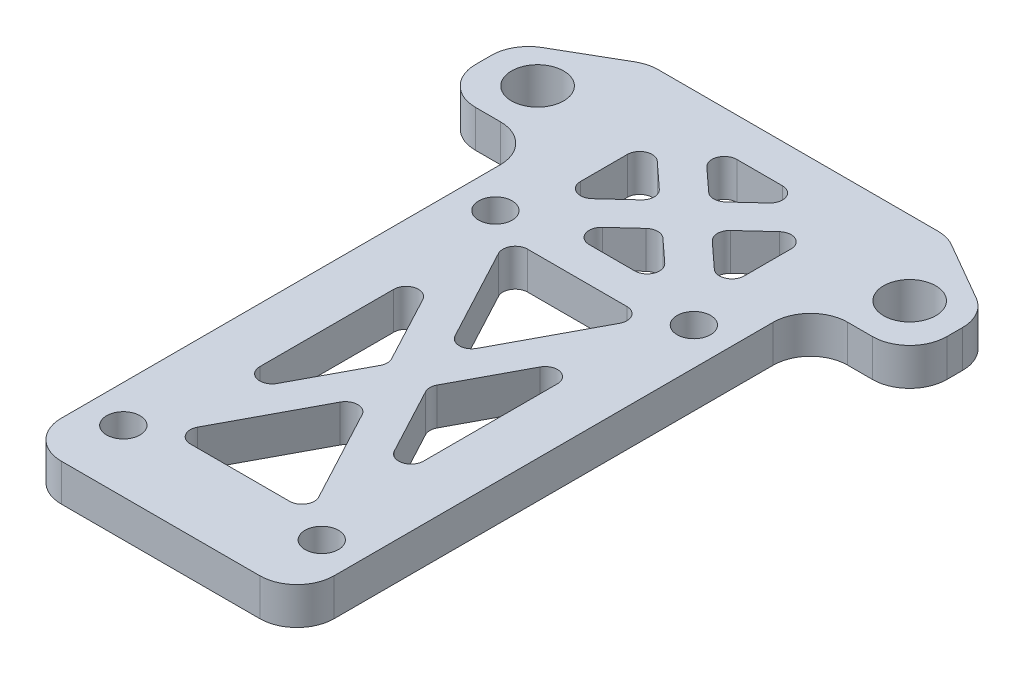
from build123d import *

# Parameters (mm, degrees)
SKETCH_1_R          = 2.1
SKETCH_1_R_2        = 1.35
EXTRUDE_1_DEPTH     = 3
CUT_EXTRUDE_1_DEPTH = 50.306794664
FILLET_R3_R         = 3
FILLET_R1_R         = 1


with BuildPart() as part:
    # 草图1 → 凸台-拉伸1 (new body)
    with BuildSketch(Plane(origin=(0, 0, 0), x_dir=(1, 0, 0), z_dir=(0, 1, 0))):
        Polygon((-12.07179677, 6), (-19, 2), (-19, -4), (-11, -4), (-11, -45.4), (11, -45.4), (11, -4), (19, -4), (19, 2), (12.07179677, 6), align=None)
        with Locations(Location((-15, 0, 0), (0, 0, 270))):
            Circle(SKETCH_1_R, mode=Mode.SUBTRACT)
        with Locations(Location((15, 0, 0), (0, 0, 270))):
            Circle(SKETCH_1_R, mode=Mode.SUBTRACT)
        with Locations(Location((-8, -10.4, 0), (0, 0, 270))):
            Circle(SKETCH_1_R_2, mode=Mode.SUBTRACT)
        with Locations(Location((-8, -40.4, 0), (0, 0, 270))):
            Circle(SKETCH_1_R_2, mode=Mode.SUBTRACT)
        with Locations(Location((8, -10.4, 0), (0, 0, 90))):
            Circle(SKETCH_1_R_2, mode=Mode.SUBTRACT)
        with Locations(Location((8, -40.4, 0), (0, 0, 90))):
            Circle(SKETCH_1_R_2, mode=Mode.SUBTRACT)
    extrude(amount=EXTRUDE_1_DEPTH)

    # 草图2 → 切除-拉伸1 (cut, through all)
    with BuildSketch(Plane(origin=(0, 3, 0), x_dir=(1, 0, 0), z_dir=(0, 1, 0))):
        Polygon((-6.6, 1.112582185), (-6.6, -7.212582185), (-2.069298303, -3.05), align=None)
        Polygon((-4.406892174, 2.9), (0, -1.148832185), (4.406892174, 2.9), align=None)
        Polygon((6.6, 1.112582185), (2.069298303, -3.05), (6.6, -7.212582185), align=None)
        Polygon((0, -4.951167815), (-4.406892174, -9), (4.406892174, -9), align=None)
        Polygon((5.666666667, -11.8), (-5.666666667, -11.8), (0, -22.425), align=None)
        Polygon((-1.586666667, -25.4), (-6.6, -16), (-6.6, -34.8), align=None)
        Polygon((5.666666667, -39), (0, -28.375), (-5.666666667, -39), align=None)
        Polygon((6.6, -16), (1.586666667, -25.4), (6.6, -34.8), align=None)
    extrude(amount=-CUT_EXTRUDE_1_DEPTH, mode=Mode.SUBTRACT)

    # R3 外缘圆角
    fillet_r3_edges = [part.edges().sort_by_distance(p)[0] for p in [
        (19, 1.5, 4),
        (11, 1.5, 4),
        (11, 1.5, 45.4),
        (-11, 1.5, 45.4),
        (-11, 1.5, 4),
        (-19, 1.5, 4),
        (-19, 1.5, -2),
        (-12.07179677, 1.5, -6),
        (12.07179677, 1.5, -6),
        (19, 1.5, -2),
    ]]
    fillet(fillet_r3_edges, radius=FILLET_R3_R)

    # R1 镂空圆角
    fillet_r1_edges = [part.edges().sort_by_distance(p)[0] for p in [
        (6.6, 1.5, 16),
        (6.6, 1.5, 34.8),
        (1.586666667, 1.5, 25.4),
        (-6.6, 1.5, 34.8),
        (-6.6, 1.5, 16),
        (-1.586666667, 1.5, 25.4),
        (5.666666667, 1.5, 39),
        (-5.666666667, 1.5, 39),
        (0, 1.5, 28.375),
        (-2.069298303, 1.5, 3.05),
        (-6.6, 1.5, 7.212582185),
        (-6.6, 1.5, -1.112582185),
        (-5.666666667, 1.5, 11.8),
        (5.666666667, 1.5, 11.8),
        (0, 1.5, 22.425),
        (0, 1.5, 4.951167815),
        (4.406892174, 1.5, 9),
        (-4.406892174, 1.5, 9),
        (4.406892174, 1.5, -2.9),
        (0, 1.5, 1.148832185),
        (-4.406892174, 1.5, -2.9),
        (6.6, 1.5, -1.112582185),
        (6.6, 1.5, 7.212582185),
        (2.069298303, 1.5, 3.05),
    ]]
    fillet(fillet_r1_edges, radius=FILLET_R1_R)


solid = part.part
